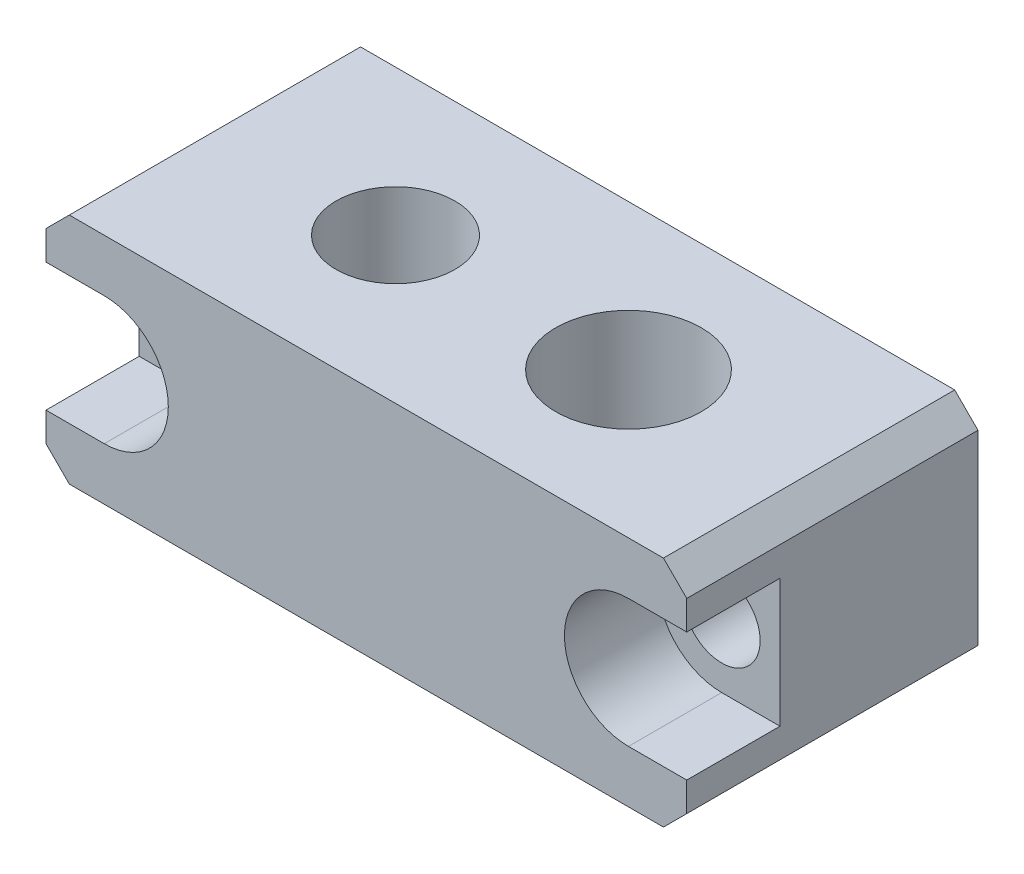
from build123d import *

# Parameters (mm, degrees)
SKETCH1_W              = 55
SKETCH1_H              = 20
BOSS_EXTRUDE1_DEPTH    = 25
CHAMFER1_SIZE          = 2
CUT_EXTRUDE1_DEPTH     = 8
HOLE1_D                = 6.6
M12_TAPPED_HOLE1_D     = 10.2
M14X1_5_TAPPED_HOLE1_D = 12.5


with BuildPart() as part:
    # Sketch1 → Boss-Extrude1 (new body)
    with BuildSketch(Plane.XY):
        with Locations((0.549312304, 3.110465116)):
            Rectangle(SKETCH1_W, SKETCH1_H)
    extrude(amount=BOSS_EXTRUDE1_DEPTH)

    # Chamfer1
    chamfer1_edges = [part.edges().sort_by_distance(p)[0] for p in [
        (-26.950687696, 13.110465116, 12.5),
        (28.049312304, 13.110465116, 12.5),
        (28.049312304, -6.889534884, 12.5),
        (-26.950687696, -6.889534884, 12.5),
    ]]
    chamfer(chamfer1_edges, length=CHAMFER1_SIZE)

    # Sketch2 → Cut-Extrude1 (cut)
    with BuildSketch(Plane.XY.offset(25)):
        with BuildLine():
            Line((-21.950687696, 8.610465116), (-26.950687696, 8.610465116))
            Line((-26.950687696, 8.610465116), (-26.950687696, -2.389534884))
            Line((-26.950687696, -2.389534884), (-21.950687696, -2.389534884))
            ThreePointArc((-21.950687696, -2.389534884), (-16.450687696, 3.110465116), (-21.950687696, 8.610465116))
        make_face()
        with BuildLine():
            Line((23.049312304, 8.610465116), (28.049312304, 8.610465116))
            Line((28.049312304, 8.610465116), (28.049312304, -2.389534884))
            Line((28.049312304, -2.389534884), (23.049312304, -2.389534884))
            ThreePointArc((23.049312304, -2.389534884), (17.549312304, 3.110465116), (23.049312304, 8.610465116))
        make_face()
    extrude(amount=-CUT_EXTRUDE1_DEPTH, mode=Mode.SUBTRACT)

    # Hole1 (through all)
    with Locations(Plane.XY.offset(17)):
        with Locations((-21.950687696, 3.110465116), (23.049312304, 3.110465116)):
            Hole(HOLE1_D / 2)

    # M12 Tapped Hole1 (through all)
    with Locations(Plane(origin=(0, -6.889534884, 0), x_dir=(-1, 0, 0), z_dir=(0, -1, 0))):
        with Locations((9.450687696, -12.5)):
            Hole(M12_TAPPED_HOLE1_D / 2)

    # M14x1.5 Tapped Hole1 (through all)
    with Locations(Plane(origin=(0, -6.889534884, 0), x_dir=(-1, 0, 0), z_dir=(0, -1, 0))):
        with Locations((-10.549312304, -12.5)):
            Hole(M14X1_5_TAPPED_HOLE1_D / 2)


solid = part.part
